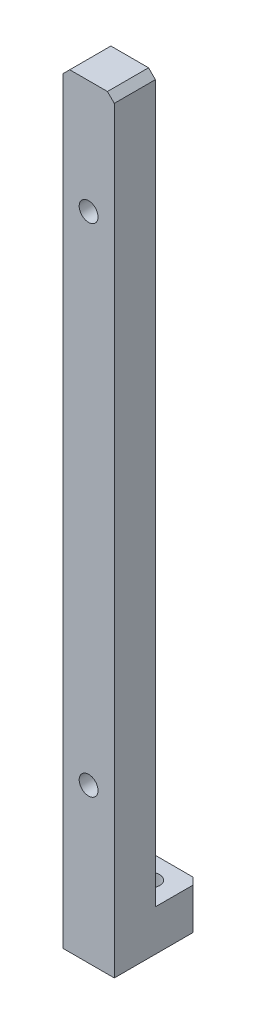
SolidWorks part; units mm, degrees
material "6061-T6"
ref_plane "Front Plane" through (0, 0, 0) normal (0, 0, 1) x (1, 0, 0)
ref_plane "Top Plane" through (0, 0, 0) normal (0, 1, 0) x (1, 0, 0)
ref_plane "Right Plane" through (0, 0, 0) normal (1, 0, 0) x (0, 0, -1)
sketch "Sketch1" plane through (0, 0, 0) normal (1, 0, 0) x (0, 0, -1)
  line L0 (0, 0) -> (25, 0)
  line L1 (25, 0) -> (25, 12)
  line L2 (25, 12) -> (12, 12)
  line L3 (12, 12) -> (12, 223.1)
  line L4 (12, 223.1) -> (0, 223.1)
  line L5 (0, 223.1) -> (0, 0)
  dimension "D1" = 25
  dimension "D2" = 12
  dimension "D3" = 12
  dimension "D4" = 223.1
extrude "Boss-Extrude1" add sketch "Sketch1" along normal blind 15
hole_wizard "CBORE for M5 Hexagon socket head cap screws1" positions "Sketch2" profile "Sketch3" counterbore size "M5" standard "GB" end condition through all
sketch "Sketch2" plane through (0, 0, -12) normal (0, 0, -1) x (-1, 0, 0)
  line L0 (-7.5, 223.1) -> (-7.5, 0) construction
  line L1 (-15, 223.1) -> (0, 223.1) construction
  line L2 (-15, 0) -> (0, 0) construction
  point P9 (-7.5, 190)
  point P11 (-7.5, 45)
  dimension "D1" = 45
  dimension "D2" = 145
sketch "Sketch3" plane through (7.5, 45, -12) normal (1, 0, 0) x (0, 1, 0)
  line L0 (0, 0) -> (0, 12)
  line L1 (0, 12) -> (2.75, 12)
  line L3 (2.75, 12) -> (2.75, 5.7)
  line L4 (2.75, 5.7) -> (5, 5.7)
  line L5 (5, 5.7) -> (5, 0)
  line L7 (5, 0) -> (0, 0)
  line L11 (0, -6.35) -> (0, 107.95) construction
  dimension "通孔孔直径" = 5.5
  dimension "通孔孔深度" = 12
  dimension "柱形沉头孔直径" = 10
  dimension "柱形沉头孔深度" = 5.7
hole_wizard "M5 Clearance Hole1" positions "Sketch4" profile "Sketch5" hole size "M5" standard "GB" end condition through all
sketch "Sketch4" plane through (0, 0, 0) normal (0, -1, 0) x (-1, 0, 0)
  line L0 (-7.5, 25) -> (-7.5, 0) construction
  line L1 (-15, 25) -> (0, 25) construction
  line L2 (-15, 0) -> (0, 0) construction
  point P9 (-7.5, 18)
  dimension "D1" = 18
sketch "Sketch5" plane through (7.5, 0, -18) normal (1, 0, 0) x (0, 0, -1)
  line L0 (0, 0) -> (0, 223.1)
  line L1 (0, 223.1) -> (2.75, 223.1)
  line L2 (2.75, 223.1) -> (2.75, 0)
  line L5 (2.75, 0) -> (0, 0)
  line L11 (0, -6.35) -> (0, 107.95) construction
  dimension "通孔孔直径" = 5.5
  dimension "通孔孔深度" = 223.1
chamfer "Chamfer1" distance 2 angle 45 4 edges at (0, 6, -25) (15, 6, -25) (0, 223.1, -6) (15, 223.1, -6)
